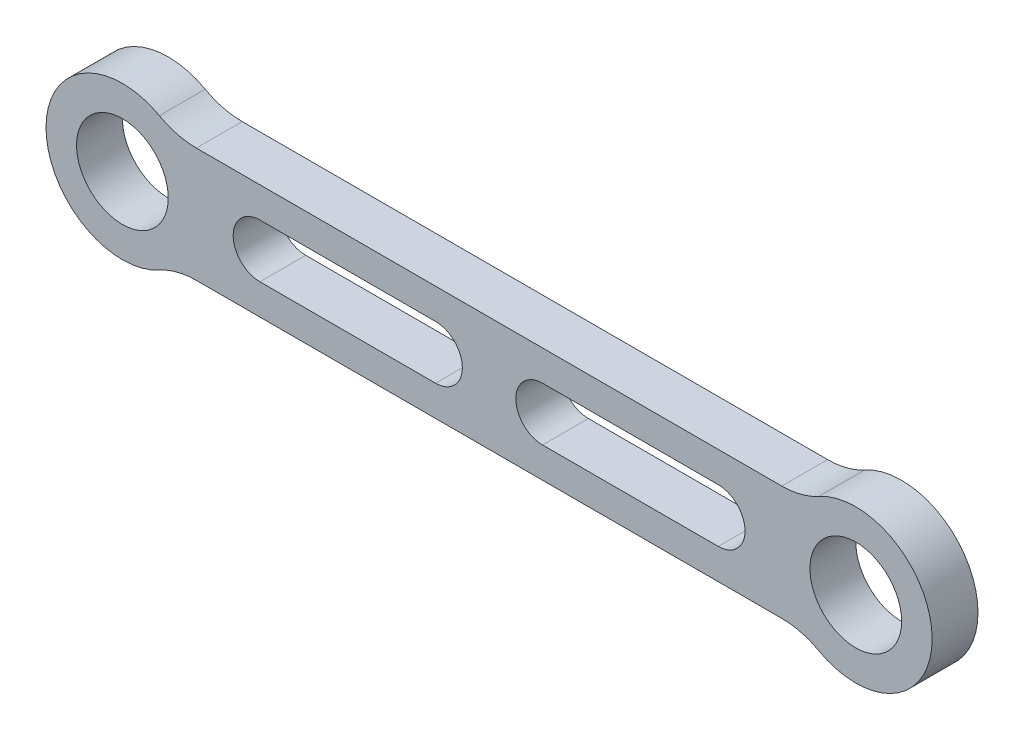
SolidWorks part; units mm, degrees
material "Thornel Mat VMA"
ref_plane "前视基准面" through (0, 0, 0) normal (0, 0, 1) x (1, 0, 0)
ref_plane "上视基准面" through (0, 0, 0) normal (0, 1, 0) x (1, 0, 0)
ref_plane "右视基准面" through (0, 0, 0) normal (1, 0, 0) x (0, 0, -1)
sketch "草图1" plane through (0, 0, 0) normal (0, 0, 1) x (1, 0, 0)
  line L0 (0, 0) -> (96, 0) construction
  line L3 (18, 0) -> (41, 0) construction
  line L6 (6.6144, 7.5) -> (89.3856, 7.5)
  line L7 (6.6144, -7.5) -> (89.3856, -7.5)
  line L8 (18, 3.5) -> (41, 3.5)
  line L9 (18, -3.5) -> (41, -3.5)
  line L10 (78, 0) -> (55, 0) construction
  line L11 (78, -3.5) -> (55, -3.5)
  line L12 (78, 3.5) -> (55, 3.5)
  line L13 (48, 7.5) -> (48, -7.5) construction
  arc A0 (6.6144, 7.5) -> (6.6144, -7.5) centre (0, 0) ccw
  arc A1 (89.3856, -7.5) -> (89.3856, 7.5) centre (96, 0) ccw
  circle A2 centre (0, 0) radius 6
  circle A3 centre (96, 0) radius 6
  arc A6 (18, 3.5) -> (18, -3.5) centre (18, 0) ccw
  arc A7 (41, -3.5) -> (41, 3.5) centre (41, 0) ccw
  arc A8 (78, -3.5) -> (78, 3.5) centre (78, 0) ccw
  arc A9 (55, 3.5) -> (55, -3.5) centre (55, 0) ccw
  point P14 (29.5, 0)
  point P20 (66.5, 0)
  dimension "D1" = 10
  dimension "D2" = 12
  dimension "D5" = 18
  dimension "D6" = 7
  dimension "D4" = 15
  dimension "D3" = 96
  dimension "D7" = 14
extrude "凸台-拉伸1" add sketch "草图1" along normal blind 6
fillet "R10 圆角1" radius 10 4 edges at (6.6144, -7.5, 3) (89.3856, -7.5, 3) (89.3856, 7.5, 3) (6.6144, 7.5, 3)
